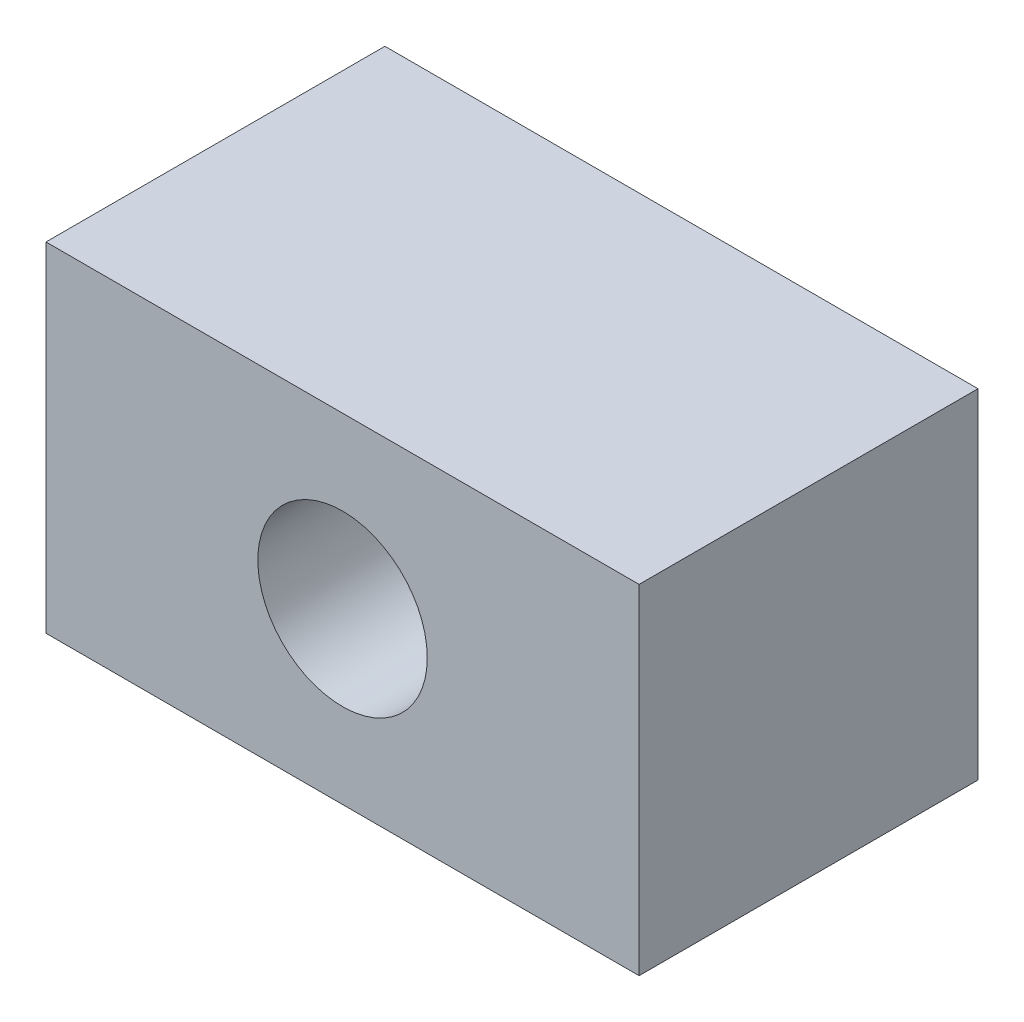
SolidWorks part; units mm, degrees
ref_plane "Front Plane" through (0, 0, 0) normal (0, 0, 1) x (1, 0, 0)
ref_plane "Top Plane" through (0, 0, 0) normal (0, 1, 0) x (1, 0, 0)
ref_plane "Right Plane" through (0, 0, 0) normal (1, 0, 0) x (0, 0, -1)
sketch "Sketch1" plane through (0, 0, 0) normal (0, 0, 1) x (1, 0, 0)
  line L1 (-17.5, 10) -> (17.5, 10)
  line L2 (-17.5, 10) -> (-17.5, -10)
  line L3 (-17.5, -10) -> (17.5, -10)
  line L4 (17.5, 10) -> (17.5, -10)
  line L5 (-17.5, 10) -> (17.5, -10) construction
  line L6 (-17.5, -10) -> (17.5, 10) construction
  circle A0 centre (0, 0) radius 5
  point P0 (0, 0)
  dimension "D3" = 10
  dimension "D1" = 35
  dimension "D2" = 20
extrude "Boss-Extrude1" add sketch "Sketch1" along normal blind 20
